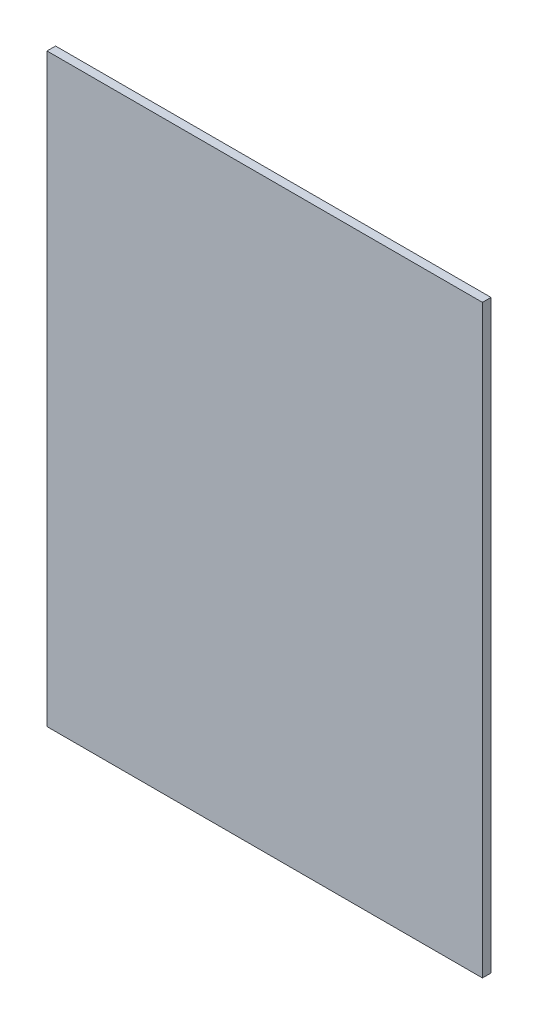
SolidWorks part; units mm, degrees
material "1060 合金"
ref_plane "Front Plane" through (0, 0, 0) normal (0, 0, 1) x (1, 0, 0)
ref_plane "Top Plane" through (0, 0, 0) normal (0, 1, 0) x (1, 0, 0)
ref_plane "Right Plane" through (0, 0, 0) normal (1, 0, 0) x (0, 0, -1)
sketch "Sketch1" plane through (0, 0, 0) normal (0, 0, 1) x (1, 0, 0)
  line L1 (0, 0) -> (101.6, 0)
  line L2 (0, 0) -> (0, 136.525)
  line L3 (0, 136.525) -> (101.6, 136.525)
  line L4 (101.6, 0) -> (101.6, 136.525)
  dimension "D1" = 136.525
  dimension "D2" = 101.6
extrude "Extrude1" add sketch "Sketch1" along normal blind 2
